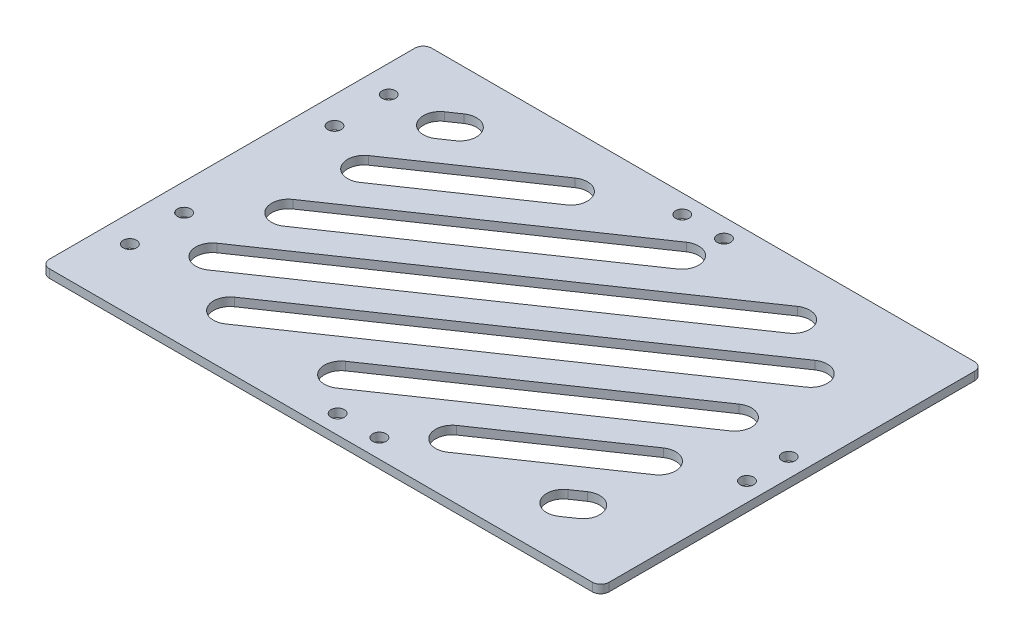
from build123d import *

# Parameters (mm, degrees)
SKETCH_1_W               = 134
SKETCH_1_H               = 91.5
SKETCH_1_R               = 1.6
EXTRUDE_1_DEPTH          = 2
CUT_EXTRUDE_2_DEPTH      = 82.982086458
CUT_EXTRUDE_2_DEPTH_BACK = 82.982086458
FILLET_R2_1_R            = 2


with BuildPart() as part:
    # 草图1 → 凸台-拉伸1 (new body)
    with BuildSketch(Plane(origin=(0, 0, 0), x_dir=(1, 0, 0), z_dir=(0, 1, 0))):
        with Locations((1, 0)):
            Rectangle(SKETCH_1_W, SKETCH_1_H)
        with Locations(Location((-59.5, 31, 0), (0, 0, 270))):
            Circle(SKETCH_1_R, mode=Mode.SUBTRACT)
        with Locations(Location((-59.5, 18, 0), (0, 0, 270))):
            Circle(SKETCH_1_R, mode=Mode.SUBTRACT)
        with Locations(Location((-59.5, -18, 0), (0, 0, 90))):
            Circle(SKETCH_1_R, mode=Mode.SUBTRACT)
        with Locations(Location((-59.5, -31, 0), (0, 0, 90))):
            Circle(SKETCH_1_R, mode=Mode.SUBTRACT)
        with Locations(Location((63.5, 3.75, 0), (0, 0, 270))):
            Circle(SKETCH_1_R, mode=Mode.SUBTRACT)
        with Locations(Location((63.5, -6.25, 0), (0, 0, 270))):
            Circle(SKETCH_1_R, mode=Mode.SUBTRACT)
        with Locations(Location((0.5, -41.25, 0), (0, 0, 270))):
            Circle(SKETCH_1_R, mode=Mode.SUBTRACT)
        with Locations(Location((10.5, -41.25, 0), (0, 0, 270))):
            Circle(SKETCH_1_R, mode=Mode.SUBTRACT)
        with Locations(Location((10.5, 41.25, 0), (0, 0, 90))):
            Circle(SKETCH_1_R, mode=Mode.SUBTRACT)
        with Locations(Location((0.5, 41.25, 0), (0, 0, 90))):
            Circle(SKETCH_1_R, mode=Mode.SUBTRACT)
    extrude(amount=EXTRUDE_1_DEPTH)

    # 草图5 → 切除-拉伸2 (cut, two sides: drawn at the far end of the back side and taken through both)
    with BuildSketch(Plane(origin=(0, 2, 0), x_dir=(1, 0, 0), z_dir=(0, 1, 0)).offset(-CUT_EXTRUDE_2_DEPTH_BACK)):
        with BuildLine():
            Line((-49.255641565, 34.099169914), (-46.471955987, 35.999970141))
            ThreePointArc((-46.471955987, 35.999970141), (-40.91297049, 34.952267774), (-41.960672856, 29.393282278))
            Line((-41.960672856, 29.393282278), (-44.744358435, 27.492482051))
            ThreePointArc((-44.744358435, 27.492482051), (-50.303343931, 28.540184417), (-49.255641565, 34.099169914))
        make_face()
        with BuildLine():
            Line((-49.255641565, 15.935756946), (-19.871985084, 35.999970141))
            ThreePointArc((-19.871985084, 35.999970141), (-14.312999587, 34.952267774), (-15.360701954, 29.393282278))
            Line((-15.360701954, 29.393282278), (-44.744358435, 9.329069084))
            ThreePointArc((-44.744358435, 9.329069084), (-50.303343931, 10.37677145), (-49.255641565, 15.935756946))
        make_face()
        with BuildLine():
            Line((-49.255641565, -2.227656021), (6.727985819, 35.999970141))
            ThreePointArc((6.727985819, 35.999970141), (12.286971315, 34.952267774), (11.239268949, 29.393282278))
            Line((11.239268949, 29.393282278), (-44.744358435, -8.834343884))
            ThreePointArc((-44.744358435, -8.834343884), (-50.303343931, -7.786641517), (-49.255641565, -2.227656021))
        make_face()
        with BuildLine():
            Line((-49.255641565, -20.391068988), (33.327956722, 35.999970141))
            ThreePointArc((33.327956722, 35.999970141), (38.886942218, 34.952267774), (37.839239852, 29.393282278))
            Line((37.839239852, 29.393282278), (-44.744358435, -26.997756851))
            ThreePointArc((-44.744358435, -26.997756851), (-50.303343931, -25.950054485), (-49.255641565, -20.391068988))
        make_face()
        with BuildLine():
            Line((-35.955656114, -29.472775472), (46.627942173, 26.918263657))
            ThreePointArc((46.627942173, 26.918263657), (52.18692767, 25.870561291), (51.139225303, 20.311575794))
            Line((51.139225303, 20.311575794), (-31.444372983, -36.079463334))
            ThreePointArc((-31.444372983, -36.079463334), (-37.00335848, -35.031760968), (-35.955656114, -29.472775472))
        make_face()
        with BuildLine():
            Line((-9.355685211, -29.472775472), (46.627942173, 8.75485069))
            ThreePointArc((46.627942173, 8.75485069), (52.18692767, 7.707148324), (51.139225303, 2.148162827))
            Line((51.139225303, 2.148162827), (-4.844402081, -36.079463334))
            ThreePointArc((-4.844402081, -36.079463334), (-10.403387577, -35.031760968), (-9.355685211, -29.472775472))
        make_face()
        with BuildLine():
            Line((17.244285692, -29.472775472), (46.627942173, -9.408562277))
            ThreePointArc((46.627942173, -9.408562277), (52.18692767, -10.456264644), (51.139225303, -16.01525014))
            Line((51.139225303, -16.01525014), (21.755568822, -36.079463334))
            ThreePointArc((21.755568822, -36.079463334), (16.196583325, -35.031760968), (17.244285692, -29.472775472))
        make_face()
        with BuildLine():
            Line((43.844256595, -29.472775472), (46.627942173, -27.571975244))
            ThreePointArc((46.627942173, -27.571975244), (52.18692767, -28.619677611), (51.139225303, -34.178663107))
            Line((51.139225303, -34.178663107), (48.355539725, -36.079463334))
            ThreePointArc((48.355539725, -36.079463334), (42.796554228, -35.031760968), (43.844256595, -29.472775472))
        make_face()
    extrude(amount=CUT_EXTRUDE_2_DEPTH + CUT_EXTRUDE_2_DEPTH_BACK, mode=Mode.SUBTRACT)

    # R2 圆角1
    fillet_r2_1_edges = [part.edges().sort_by_distance(p)[0] for p in [
        (-66, 1, -45.75),
        (68, 1, -45.75),
        (68, 1, 45.75),
        (-66, 1, 45.75),
    ]]
    fillet(fillet_r2_1_edges, radius=FILLET_R2_1_R)


solid = part.part
